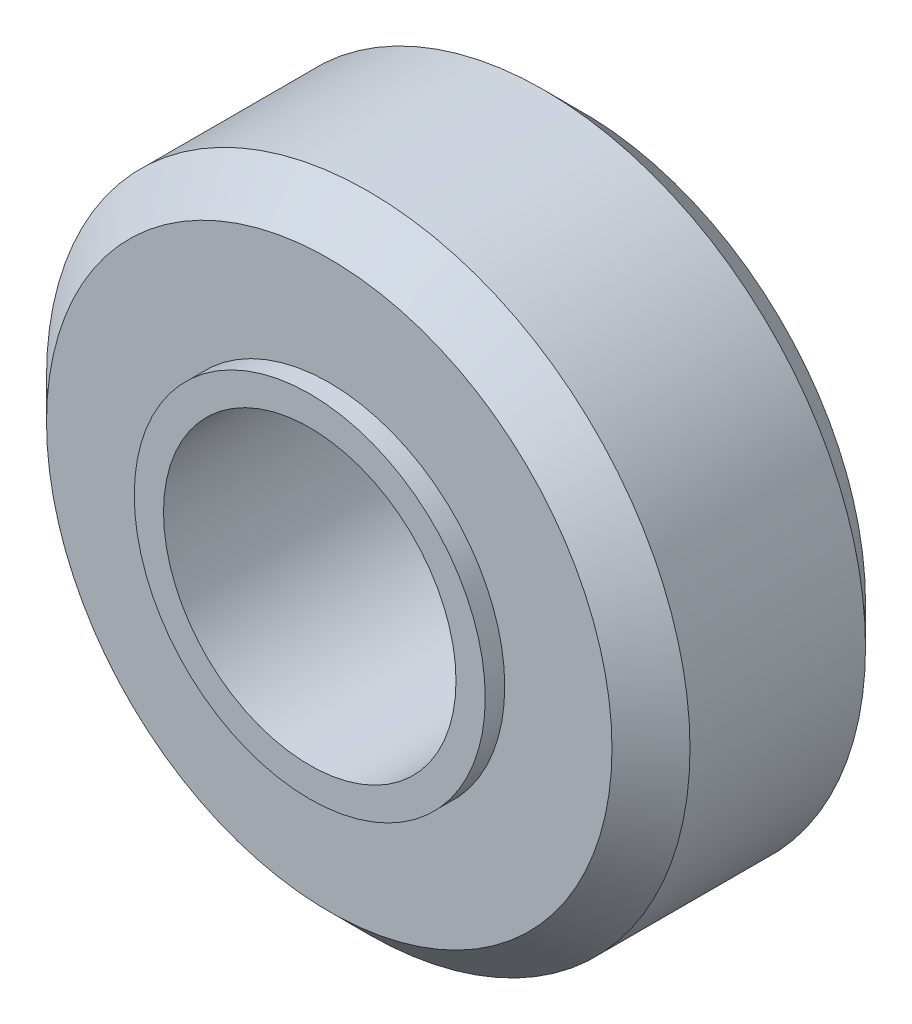
from build123d import *

# Parameters (mm, degrees)
SKETCH_1_R      = 16.5
SKETCH_1_R_2    = 7.5
EXTRUDE_1_DEPTH = 10
SKETCH_2_R      = 9
SKETCH_2_R_2    = 7.5
EXTRUDE_2_DEPTH = 1
EXTRUDE_START   = 3
SKETCH_3_R      = 16.5
EXTRUDE_3_DEPTH = 3
CHAMFER_1_SIZE  = 2


with BuildPart() as part:
    # 草图1 → 凸台-拉伸1 (new body)
    with BuildSketch(Plane.XY):
        Circle(SKETCH_1_R)
        Circle(SKETCH_1_R_2, mode=Mode.SUBTRACT)
    extrude(amount=EXTRUDE_1_DEPTH)

    # 草图2 → 凸台-拉伸2 (add)
    with BuildSketch(Plane.XY.offset(10)):
        Circle(SKETCH_2_R)
        Circle(SKETCH_2_R_2, mode=Mode.SUBTRACT)
    extrude(amount=EXTRUDE_2_DEPTH)

    # 草图3 → 凸台-拉伸3 (add)
    with BuildSketch(Plane(origin=(0, 0, 0), x_dir=(-1, 0, 0), z_dir=(0, 0, -1)).offset(EXTRUDE_START)):
        Circle(SKETCH_3_R)
    extrude(amount=-EXTRUDE_3_DEPTH)

    # 倒角1
    chamfer_1_edges = [part.edges().sort_by_distance(p)[0] for p in [
        (16.5, 0, -3),
        (-16.5, 0, 10),
    ]]
    chamfer(chamfer_1_edges, length=CHAMFER_1_SIZE)


solid = part.part
